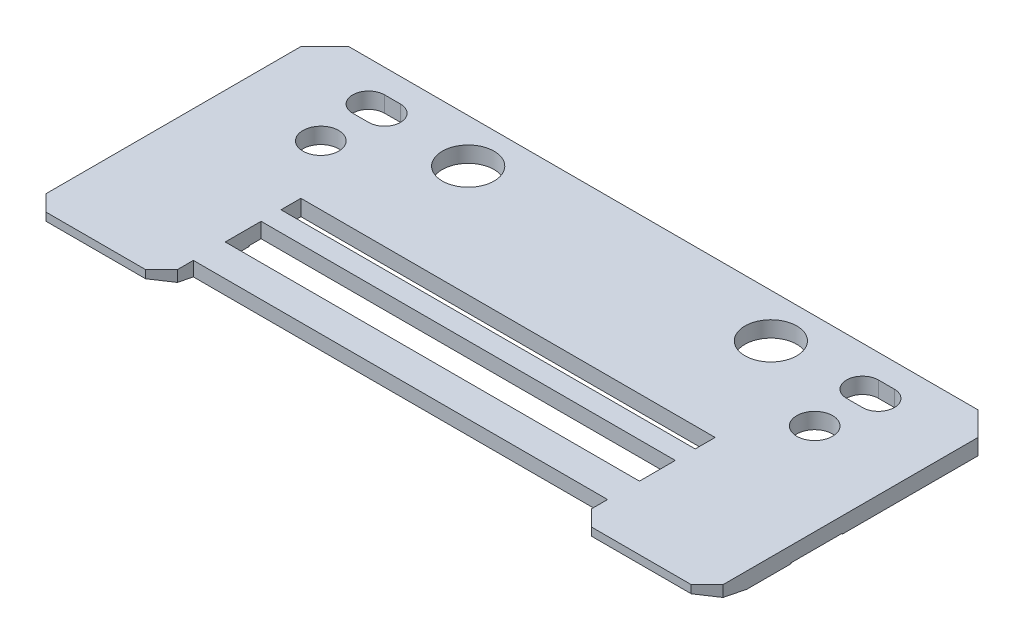
from build123d import *

# Parameters (mm, degrees)
SKETCH1_W           = 85
SKETCH1_H           = 45
BOSS_EXTRUDE1_DEPTH = 2
SKETCH2_W           = 52
SKETCH2_H           = 12
SKETCH2_H_2         = 4.5
SKETCH2_H_3         = 2.5
SKETCH2_H_4         = 13.8
CUT_EXTRUDE1_DEPTH  = 10
SKETCH3_W           = 85
SKETCH3_H           = 13.8
CUT_EXTRUDE2_DEPTH  = 10
SKETCH5_W           = 85
SKETCH5_H           = 5.5
CUT_EXTRUDE4_DEPTH  = 0.1
CHAMFER2_SIZE       = 0.5
CHAMFER2_SIZE2      = 2
CHAMFER3_SIZE       = 2
CHAMFER3_SIZE2      = 0.5
SKETCH8_W           = 85
SKETCH8_H           = 13.8
BOSS_EXTRUDE2_DEPTH = 2
CHAMFER4_SIZE       = 3
SKETCH6_R           = 2
CUT_EXTRUDE5_DEPTH  = 10
CUT_EXTRUDE6_DEPTH  = 6
SKETCH9_R           = 3.25
CUT_EXTRUDE8_DEPTH  = 10
SKETCH4_R           = 2.25
CUT_EXTRUDE3_DEPTH  = 10
SKETCH10_W          = 85
SKETCH10_H          = 8
CUT_EXTRUDE9_DEPTH  = 10
CHAMFER5_SIZE       = 1
CHAMFER5_SIZE2      = 5
CHAMFER6_SIZE       = 2


with BuildPart() as part:
    # Sketch1 → Boss-Extrude1 (new body)
    with BuildSketch(Plane(origin=(0, 0, 0), x_dir=(1, 0, 0), z_dir=(0, 1, 0))):
        Rectangle(SKETCH1_W, SKETCH1_H)
    extrude(amount=BOSS_EXTRUDE1_DEPTH)

    # Sketch2 → Cut-Extrude1 (cut)
    with BuildSketch(Plane(origin=(0, 2, 0), x_dir=(1, 0, 0), z_dir=(0, 1, 0))):
        with Locations((0, -16.5)):
            Rectangle(SKETCH2_W, SKETCH2_H)
        with Locations((0, -4.25)):
            Rectangle(SKETCH2_W, SKETCH2_H_2)
        with Locations((0, 1.75)):
            Rectangle(SKETCH2_W, SKETCH2_H_3)
        with Locations((0, 15.6)):
            Rectangle(SKETCH2_W, SKETCH2_H_4)
    extrude(amount=-CUT_EXTRUDE1_DEPTH, mode=Mode.SUBTRACT)

    # Sketch3 → Cut-Extrude2 (cut)
    with BuildSketch(Plane(origin=(0, 2, 0), x_dir=(1, 0, 0), z_dir=(0, 1, 0))):
        with Locations((0, 15.6)):
            Rectangle(SKETCH3_W, SKETCH3_H)
    extrude(amount=-CUT_EXTRUDE2_DEPTH, mode=Mode.SUBTRACT)

    # Sketch5 → Cut-Extrude4 (cut)
    with BuildSketch(Plane.XZ):
        with Locations((0, 0.75)):
            Rectangle(SKETCH5_W, SKETCH5_H)
    extrude(amount=-CUT_EXTRUDE4_DEPTH, mode=Mode.SUBTRACT)

    # Chamfer2
    chamfer2_edges = [part.edges().sort_by_distance(p)[0] for p in [
        (42.5, 0.05, 3.5),
    ]]
    chamfer2_side = [part.faces().sort_by_distance(p)[0] for p in [
        (42.5, 1.008447858, 6.954688763),
    ]]
    chamfer(chamfer2_edges, length=CHAMFER2_SIZE, length2=CHAMFER2_SIZE2, reference=chamfer2_side[0])

    # Chamfer3
    chamfer3_edges = [part.edges().sort_by_distance(p)[0] for p in [
        (42.5, 0.05, -2),
    ]]
    chamfer3_side = [part.faces().sort_by_distance(p)[0] for p in [
        (34.25, 0.05, -2),
    ]]
    chamfer(chamfer3_edges, length=CHAMFER3_SIZE, length2=CHAMFER3_SIZE2, reference=chamfer3_side[0])

    # Sketch8 → Boss-Extrude2 (add)
    with BuildSketch(Plane(origin=(0, 2, 0), x_dir=(1, 0, 0), z_dir=(0, 1, 0))):
        with Locations((0, 15.6)):
            Rectangle(SKETCH8_W, SKETCH8_H)
    extrude(amount=-BOSS_EXTRUDE2_DEPTH)

    # Chamfer4
    chamfer4_edges = [part.edges().sort_by_distance(p)[0] for p in [
        (-42.5, 1, -22.5),
        (42.5, 1, -22.5),
    ]]
    chamfer(chamfer4_edges, length=CHAMFER4_SIZE)

    # Sketch6 → Cut-Extrude5 (cut)
    with BuildSketch(Plane(origin=(0, 2, 0), x_dir=(1, 0, 0), z_dir=(0, 1, 0))):
        with Locations(Location((-31, 17.5, 0), (0, 0, 270))):
            Circle(SKETCH6_R)
        with Locations(Location((31, 17.5, 0), (0, 0, 270))):
            Circle(SKETCH6_R)
    extrude(amount=-CUT_EXTRUDE5_DEPTH, mode=Mode.SUBTRACT)

    # Sketch7 → Cut-Extrude6 (cut)
    with BuildSketch(Plane(origin=(0, 2, 0), x_dir=(1, 0, 0), z_dir=(0, 1, 0))):
        with BuildLine():
            Line((32, 15.5), (30, 15.5))
            ThreePointArc((30, 15.5), (28, 17.5), (30, 19.5))
            Line((30, 19.5), (32, 19.5))
            ThreePointArc((32, 19.5), (34, 17.5), (32, 15.5))
        make_face()
        with BuildLine():
            Line((-32, 15.5), (-30, 15.5))
            ThreePointArc((-30, 15.5), (-28, 17.5), (-30, 19.5))
            Line((-30, 19.5), (-32, 19.5))
            ThreePointArc((-32, 19.5), (-34, 17.5), (-32, 15.5))
        make_face()
    extrude(amount=-CUT_EXTRUDE6_DEPTH, mode=Mode.SUBTRACT)

    # Sketch9 → Cut-Extrude8 (cut)
    with BuildSketch(Plane(origin=(0, 2, 0), x_dir=(1, 0, 0), z_dir=(0, 1, 0))):
        with Locations(Location((-19, 17, 0), (0, 0, 270))):
            Circle(SKETCH9_R)
        with Locations(Location((19, 17, 0), (0, 0, 270))):
            Circle(SKETCH9_R)
    extrude(amount=-CUT_EXTRUDE8_DEPTH, mode=Mode.SUBTRACT)

    # Sketch4 → Cut-Extrude3 (cut)
    with BuildSketch(Plane(origin=(0, 2, 0), x_dir=(1, 0, 0), z_dir=(0, 1, 0))):
        with Locations(Location((-31, 10.5, 0), (0, 0, 270))):
            Circle(SKETCH4_R)
        with Locations(Location((31, 10.5, 0), (0, 0, 270))):
            Circle(SKETCH4_R)
    extrude(amount=-CUT_EXTRUDE3_DEPTH, mode=Mode.SUBTRACT)

    # Sketch10 → Cut-Extrude9 (cut)
    with BuildSketch(Plane(origin=(0, 2, 0), x_dir=(1, 0, 0), z_dir=(0, 1, 0))):
        with Locations((0, -18.5)):
            Rectangle(SKETCH10_W, SKETCH10_H)
    extrude(amount=-CUT_EXTRUDE9_DEPTH, mode=Mode.SUBTRACT)

    # Chamfer5
    chamfer5_edges = [part.edges().sort_by_distance(p)[0] for p in [
        (-34.25, 0, 14.5),
    ]]
    chamfer5_side = [part.faces().sort_by_distance(p)[0] for p in [
        (-34.25, 1, 14.5),
    ]]
    chamfer(chamfer5_edges, length=CHAMFER5_SIZE, length2=CHAMFER5_SIZE2, reference=chamfer5_side[0])

    # Chamfer6
    chamfer6_edges = [part.edges().sort_by_distance(p)[0] for p in [
        (-26, 1.5, 14.5),
        (-42.5, 1.5, 14.5),
        (26, 1.5, 14.5),
        (42.5, 1.5, 14.5),
    ]]
    chamfer(chamfer6_edges, length=CHAMFER6_SIZE)


solid = part.part
